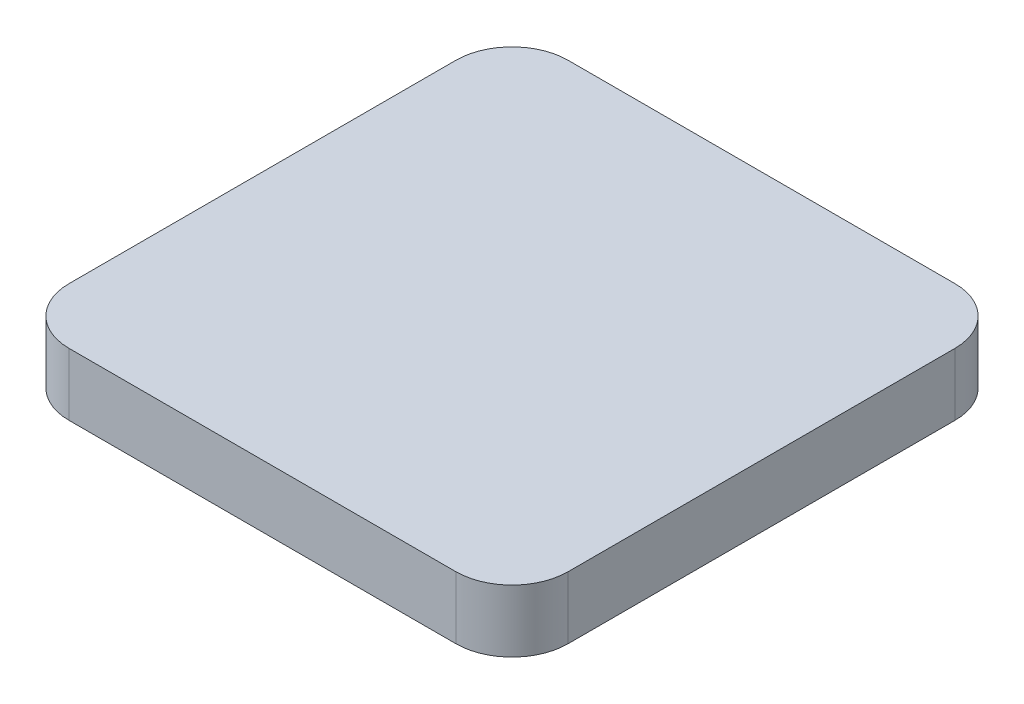
from build123d import *

# Parameters (mm, degrees)
SKETCH_1_W      = 40
SKETCH_1_H      = 40
EXTRUDE_1_DEPTH = 2.5
FILLET_1_R      = 4.5


with BuildPart() as part:
    # 草图1 → 凸台-拉伸1 (new, symmetric)
    with BuildSketch(Plane(origin=(0, 0, 0), x_dir=(1, 0, 0), z_dir=(0, 1, 0))):
        Rectangle(SKETCH_1_W, SKETCH_1_H)
    extrude(amount=EXTRUDE_1_DEPTH, both=True)

    # 圆角1
    fillet_1_edges = [part.edges().sort_by_distance(p)[0] for p in [
        (20, 0, 20),
        (-20, 0, 20),
        (-20, 0, -20),
        (20, 0, -20),
    ]]
    fillet(fillet_1_edges, radius=FILLET_1_R)


solid = part.part
